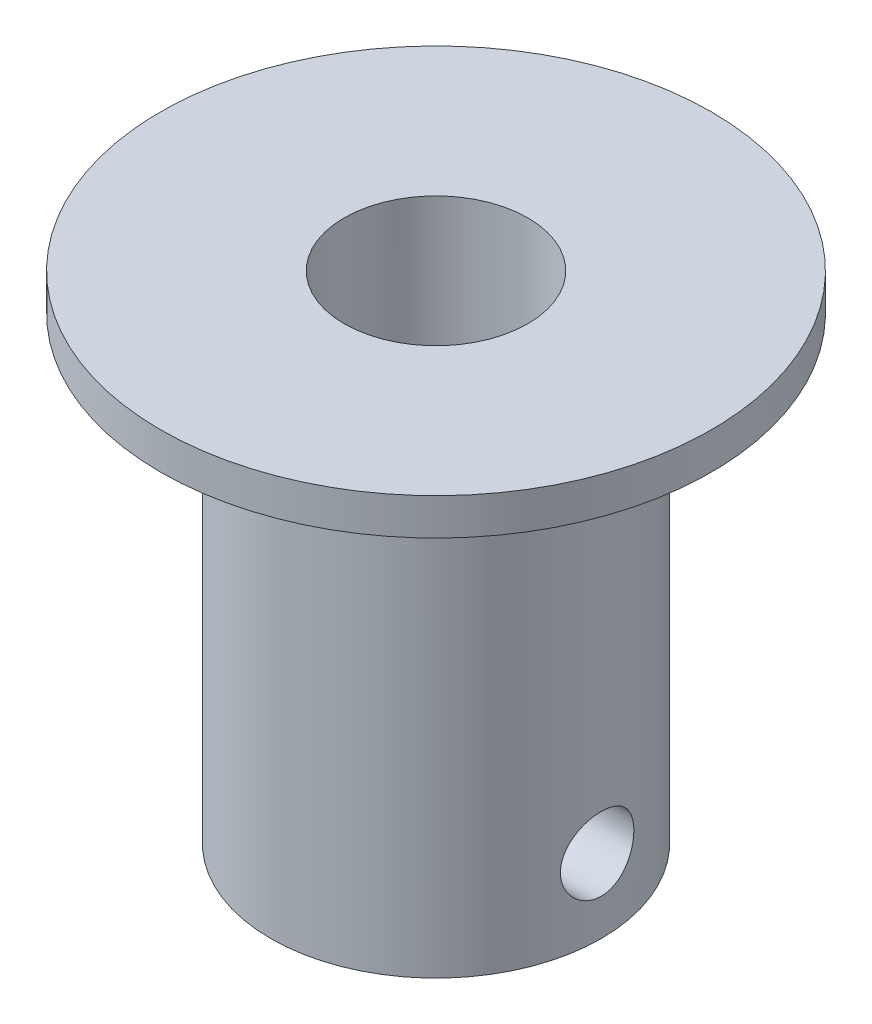
SolidWorks part; units mm, degrees
material "普通碳钢"
ref_plane "Front Plane" through (0, 0, 0) normal (0, 0, 1) x (1, 0, 0)
ref_plane "Top Plane" through (0, 0, 0) normal (0, 1, 0) x (1, 0, 0)
ref_plane "Right Plane" through (0, 0, 0) normal (1, 0, 0) x (0, 0, -1)
sketch "Sketch2" plane through (0, 0, 0) normal (0, 1, 0) x (1, 0, 0)
  circle A0 centre (0, 0) radius 25
  circle A1 centre (0, 0) radius 75
  dimension "D1" = 50
  dimension "D2" = 150
extrude "Boss-Extrude1" add sketch "Sketch2" along normal blind 10
sketch "Sketch3" plane through (0, 0, 0) normal (0, -1, 0) x (1, 0, 0)
  circle A0 centre (0, 0) radius 25
  circle A1 centre (0, 0) radius 45
extrude "Boss-Extrude2" add sketch "Sketch3" along normal blind 125
sketch "Sketch4" plane through (0, 0, 0) normal (1, 0, 0) x (0, 0, -1)
  line L0 (-45, -125) -> (45, -125) construction
  circle A0 centre (0, -105) radius 10
  dimension "D1" = 20
  dimension "D2" = 20
extrude "Cut-Extrude1" cut sketch "Sketch4" against normal through all both and the other way through all
ref_plane "Plane1" through (0, 0, 45) normal (0, 0, 1) x (1, 0, 0)
